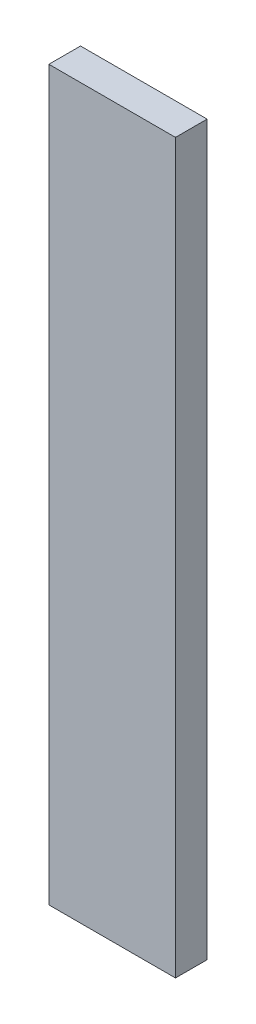
SolidWorks part; units mm, degrees
ref_plane "Front Plane" through (0, 0, 0) normal (0, 0, 1) x (1, 0, 0)
ref_plane "Top Plane" through (0, 0, 0) normal (0, 1, 0) x (1, 0, 0)
ref_plane "Right Plane" through (0, 0, 0) normal (1, 0, 0) x (0, 0, -1)
sketch "Sketch1" plane through (0, 0, 0) normal (0, 0, 1) x (1, 0, 0)
  line L1 (40, -230) -> (-40, -230)
  line L2 (40, -230) -> (40, 230)
  line L3 (40, 230) -> (-40, 230)
  line L4 (-40, -230) -> (-40, 230)
  line L5 (40, -230) -> (-40, 230) construction
  line L6 (40, 230) -> (-40, -230) construction
  point P0 (0, 0)
  dimension "D1" = 80
  dimension "D2" = 460
extrude "Boss-Extrude1" add sketch "Sketch1" along normal blind 20
